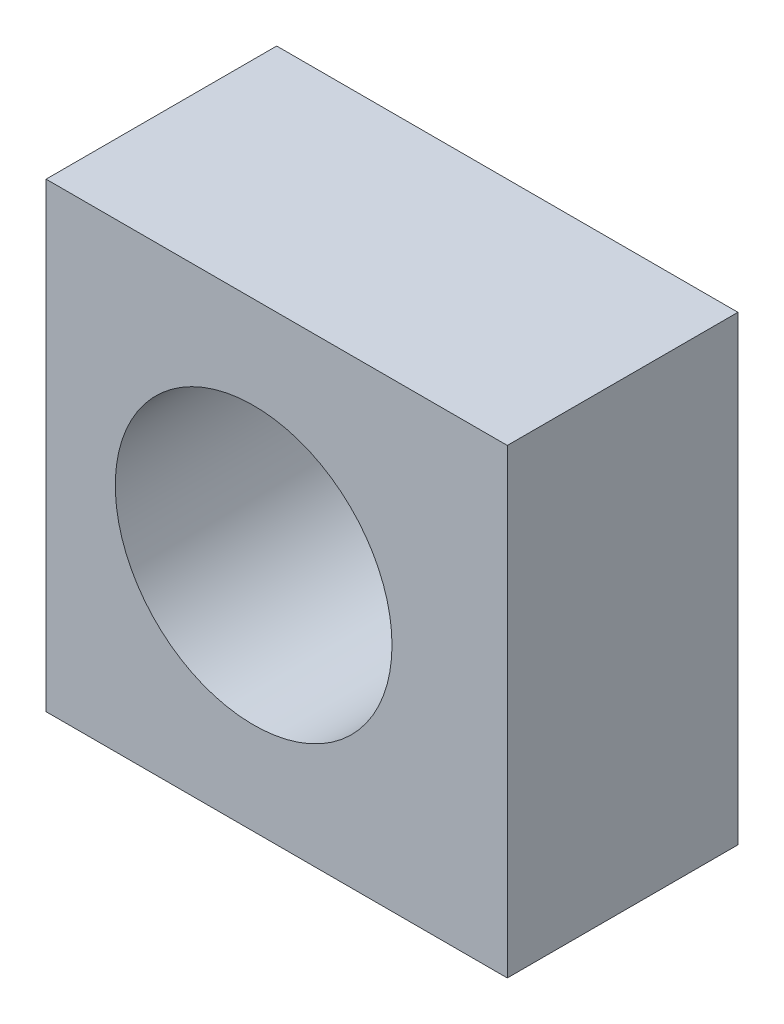
SolidWorks part; units mm, degrees
material "1023 Carbon steel plate (SS)"
ref_plane "Front Plane" through (0, 0, 0) normal (0, 0, 1) x (1, 0, 0)
ref_plane "Top Plane" through (0, 0, 0) normal (0, 1, 0) x (1, 0, 0)
ref_plane "Right Plane" through (0, 0, 0) normal (1, 0, 0) x (0, 0, -1)
sketch "Sketch1" plane through (0, 0, 0) normal (0, 0, 1) x (1, 0, 0)
  line L1 (-10, 10) -> (10, 10)
  line L2 (-10, 10) -> (-10, -10)
  line L3 (-10, -10) -> (10, -10)
  line L4 (10, 10) -> (10, -10)
  line L5 (-10, 10) -> (10, -10) construction
  line L6 (-10, -10) -> (10, 10) construction
  circle A0 centre (-1, 0) radius 6
  point P0 (-1, 0)
  dimension "D3" = 12
  dimension "D4" = 10
  dimension "D5" = 9
  dimension "D1" = 20
  dimension "D2" = 20
extrude "Boss-Extrude1" add sketch "Sketch1" along normal blind 10
